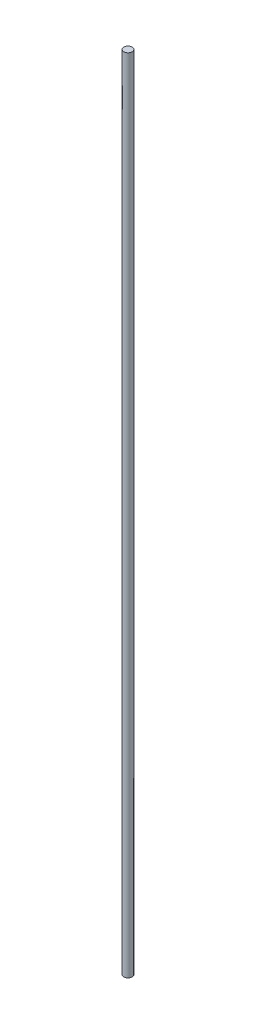
SolidWorks part; units mm, degrees
material "黄铜"
ref_plane "Front Plane" through (0, 0, 0) normal (0, 0, 1) x (1, 0, 0)
ref_plane "Top Plane" through (0, 0, 0) normal (0, 1, 0) x (1, 0, 0)
ref_plane "Right Plane" through (0, 0, 0) normal (1, 0, 0) x (0, 0, -1)
sketch "Sketch1" plane through (0, 0, 0) normal (0, 0, 1) x (1, 0, 0)
  line L1 (0, 0) -> (-0.25, 0)
  line L2 (0, 0) -> (0, 48)
  line L3 (0, 48) -> (-0.25, 48)
  line L4 (-0.25, 0) -> (-0.25, 48)
  dimension "D1" = 48
  dimension "D2" = 0.25
revolve "Revolve1" add sketch "Sketch1" angle 360 about L2
